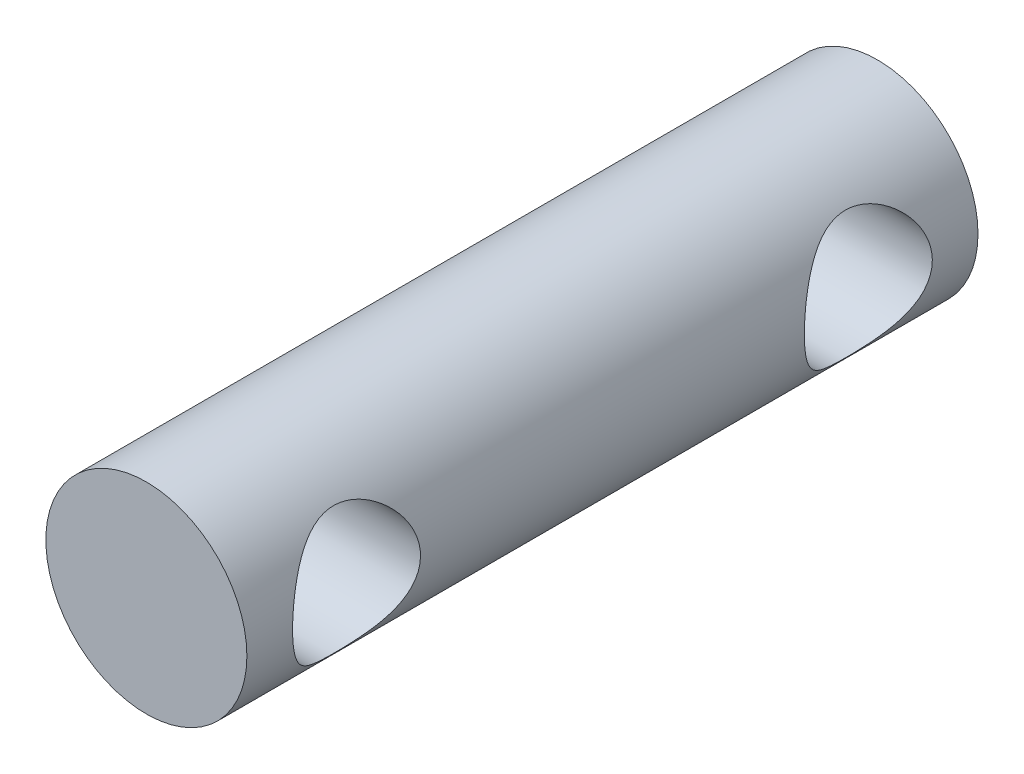
from build123d import *

# Parameters (mm, degrees)
SKETCH_1_R          = 5.5
EXTRUDE_1_DEPTH     = 20
SKETCH_2_R          = 3.5
CUT_EXTRUDE_1_DEPTH = 20


with BuildPart() as part:
    # 草图1 → 凸台-拉伸1 (new, symmetric)
    with BuildSketch(Plane.XY):
        Circle(SKETCH_1_R)
    extrude(amount=EXTRUDE_1_DEPTH, both=True)

    # 草图2 → 切除-拉伸1 (cut, symmetric)
    with BuildSketch(Plane(origin=(0, 0, 0), x_dir=(0, 0, -1), z_dir=(1, 0, 0))):
        with Locations(Location((-14, 0, 0), (0, 0, 180.000000005))):
            Circle(SKETCH_2_R)
        with Locations(Location((14, 0, 0), (0, 0, 180.000000005))):
            Circle(SKETCH_2_R)
    extrude(amount=CUT_EXTRUDE_1_DEPTH, both=True, mode=Mode.SUBTRACT)


solid = part.part
